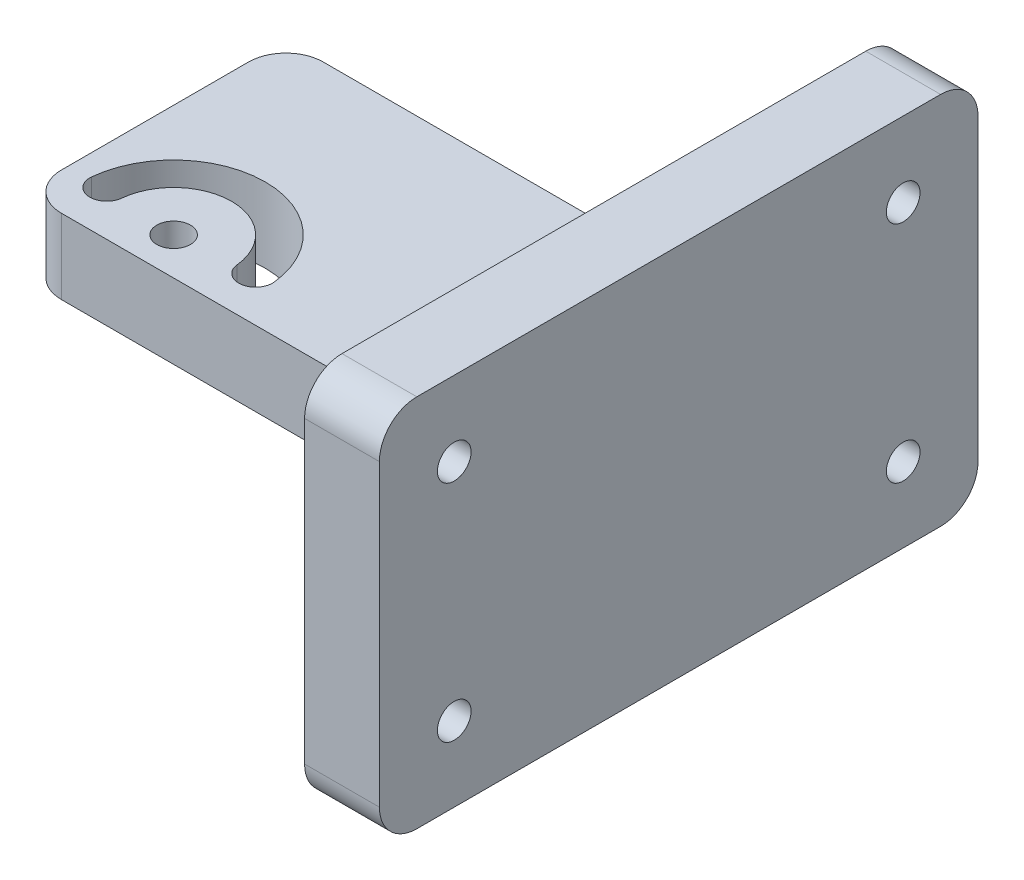
SolidWorks part; units mm, degrees
ref_plane "前视基准面" through (0, 0, 0) normal (0, 0, 1) x (1, 0, 0)
ref_plane "上视基准面" through (0, 0, 0) normal (0, 1, 0) x (1, 0, 0)
ref_plane "右视基准面" through (0, 0, 0) normal (1, 0, 0) x (0, 0, -1)
sketch "草图1" plane through (0, 0, 0) normal (0, 1, 0) x (1, 0, 0)
  line L1 (-30, 17.5) -> (30, 17.5)
  line L2 (-30, 17.5) -> (-30, -17.5)
  line L3 (-30, -17.5) -> (30, -17.5)
  line L4 (30, 17.5) -> (30, -17.5)
  line L5 (-30, 17.5) -> (30, -17.5) construction
  line L6 (-30, -17.5) -> (30, 17.5) construction
  point P0 (0, 0)
  dimension "D1" = 60
  dimension "D2" = 35
extrude "凸台-拉伸1" add sketch "草图1" along normal mid plane 10
sketch "草图2" plane through (0, -5, 0) normal (0, -1, 0) x (1, 0, 0)
  line L0 (-15, 17.5) -> (-15, -17.5) construction
  line L1 (-30, 17.5) -> (30, 17.5) construction
  line L2 (-30, -17.5) -> (-30, 17.5) construction
  circle A0 centre (-15, 12.5) radius 2.25
  circle A1 centre (-15, 2.5) radius 2.25
  dimension "D3" = 4.5
  dimension "D1" = 10
  dimension "D2" = 5
  dimension "D4" = 15
extrude "切除-拉伸1" cut sketch "草图2" against normal through all
sketch "草图3" plane through (0, -5, 0) normal (0, -1, 0) x (1, 0, 0)
  circle A0 centre (-15, 12.5) radius 10 construction
  arc A7 (-27.1886, 11.275) -> (-2.8114, 11.275) centre (-15, 12.5) ccw
  arc A8 (-22.7112, 11.725) -> (-7.2888, 11.725) centre (-15, 12.5) ccw
  circle A9 centre (-15, 2.5) radius 2.25 construction
  arc A10 (-2.8114, 11.275) -> (-7.2888, 11.725) centre (-5.0501, 11.5) ccw
  arc A11 (-22.7112, 11.725) -> (-27.1886, 11.275) centre (-24.9499, 11.5) ccw
  dimension "D1" = 1
extrude "切除-拉伸2" cut sketch "草图3" against normal through all
sketch "草图5" plane through (30, 0, 0) normal (1, 0, 0) x (0, 0, -1)
  line L1 (-40, 25) -> (40, 25)
  line L2 (-40, 25) -> (-40, -25)
  line L3 (-40, -25) -> (40, -25)
  line L4 (40, 25) -> (40, -25)
  line L5 (-40, 25) -> (40, -25) construction
  line L6 (-40, -25) -> (40, 25) construction
  point P0 (0, 0)
  dimension "D1" = 80
  dimension "D2" = 50
extrude "凸台-拉伸3" add sketch "草图5" along normal blind 10
hole_wizard "M4 六角凹头螺钉的柱形沉头孔1" positions "草图6" profile "草图7" counterbore size "M4" standard "ISO" end condition through all
sketch "草图6" plane through (30, 0, 0) normal (-1, 0, 0) x (0, 0, 1)
  line L0 (0, 0) -> (40, 0) construction
  line L1 (40, 25) -> (40, -25) construction
  line L3 (0, 0) -> (0, 25) construction
  line L4 (-40, 25) -> (40, 25) construction
  point P0 (30, 15)
  point P2 (-30, 15)
  point P4 (-30, -15)
  point P6 (30, -15)
  dimension "D1" = 60
  dimension "D2" = 30
sketch "草图7" plane through (30, 15, 30) normal (0, 1, 0) x (0, 0, 1)
  line L0 (0, 0) -> (0, 10)
  line L1 (0, 10) -> (2.25, 10)
  line L3 (2.25, 10) -> (2.25, 4.4)
  line L4 (2.25, 4.4) -> (4, 4.4)
  line L5 (4, 4.4) -> (4, 0)
  line L7 (4, 0) -> (0, 0)
  line L11 (0, -6.35) -> (0, 107.95) construction
  dimension "通孔孔直径" = 4.5
  dimension "通孔孔深度" = 10
  dimension "柱形沉头孔直径" = 8
  dimension "柱形沉头孔深度" = 4.4
fillet "圆角1" radius 5 6 edges at (-30, 0, 17.5) (-30, 0, -17.5) (35, -25, 40) (35, 25, 40) (35, -25, -40) (35, 25, -40)
